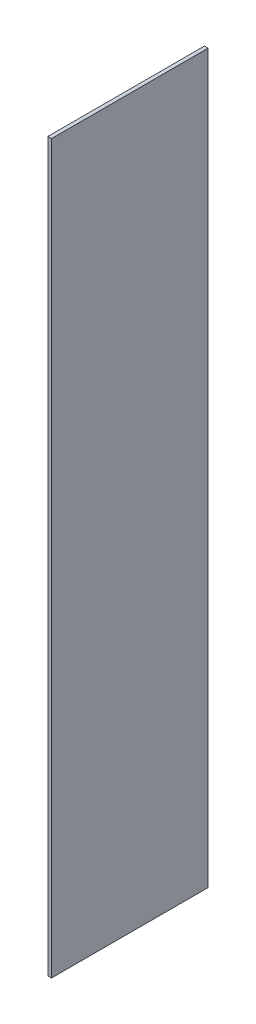
from build123d import *

# Parameters (mm, degrees)
SKETCH1_W           = 1.5
SKETCH1_H           = 297
BOSS_EXTRUDE1_DEPTH = 32


with BuildPart() as part:
    # Sketch1 → Boss-Extrude1 (new, symmetric)
    with BuildSketch(Plane.XY):
        Rectangle(SKETCH1_W, SKETCH1_H)
    extrude(amount=BOSS_EXTRUDE1_DEPTH, both=True)


solid = part.part
